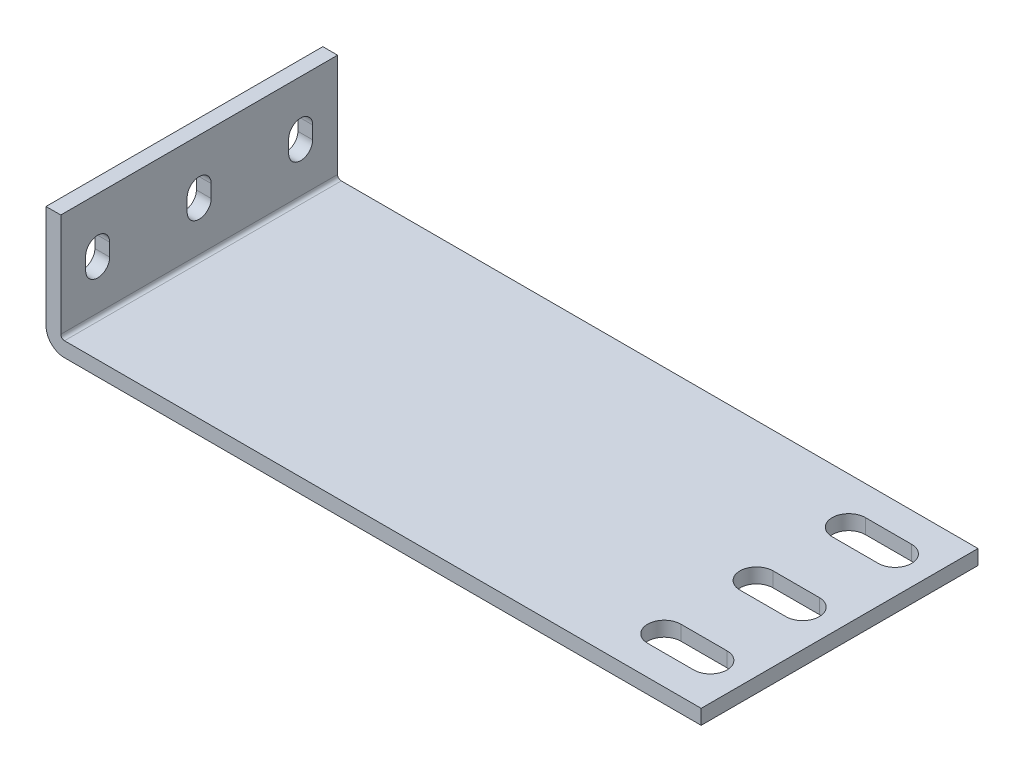
from build123d import *

# Parameters (mm, degrees)
EXTRUDE_1_DEPTH     = 150
CUT_EXTRUDE_1_DEPTH = 150
CUT_EXTRUDE_2_DEPTH = 150


with BuildPart() as part:
    # 草图1 → 凸台-拉伸1 (new body)
    with BuildSketch(Plane.XY):
        with BuildLine():
            Line((0, 0), (0, -56))
            ThreePointArc((0, -56), (2.928932188, -63.071067812), (10, -66))
            Line((10, -66), (355, -66))
            Line((355, -66), (355, -58))
            Line((355, -58), (10, -58))
            ThreePointArc((10, -58), (8.585786438, -57.414213562), (8, -56))
            Line((8, -56), (8, 0))
            Line((8, 0), (0, 0))
        make_face()
    extrude(amount=EXTRUDE_1_DEPTH)

    # 草图2 → 切除-拉伸1 (cut)
    with BuildSketch(Plane.ZY):
        with BuildLine():
            Line((26.5, -26), (26.5, -33))
            ThreePointArc((26.5, -33), (20, -39.5), (13.5, -33))
            Line((13.5, -33), (13.5, -26))
            ThreePointArc((13.5, -26), (20, -19.5), (26.5, -26))
        make_face()
        with BuildLine():
            Line((81.5, -26), (81.5, -33))
            ThreePointArc((81.5, -33), (75, -39.5), (68.5, -33))
            Line((68.5, -33), (68.5, -26))
            ThreePointArc((68.5, -26), (75, -19.5), (81.5, -26))
        make_face()
        with BuildLine():
            Line((136.5, -26), (136.5, -33))
            ThreePointArc((136.5, -33), (130, -39.5), (123.5, -33))
            Line((123.5, -33), (123.5, -26))
            ThreePointArc((123.5, -26), (130, -19.5), (136.5, -26))
        make_face()
    extrude(amount=-CUT_EXTRUDE_1_DEPTH, mode=Mode.SUBTRACT)

    # 草图3 → 切除-拉伸2 (cut)
    with BuildSketch(Plane(origin=(0, -58, 0), x_dir=(1, 0, 0), z_dir=(0, 1, 0))):
        with BuildLine():
            Line((310, -16), (335, -16))
            ThreePointArc((335, -16), (344, -25), (335, -34))
            Line((335, -34), (310, -34))
            ThreePointArc((310, -34), (301, -25), (310, -16))
        make_face()
        with BuildLine():
            Line((310, -66), (335, -66))
            ThreePointArc((335, -66), (344, -75), (335, -84))
            Line((335, -84), (310, -84))
            ThreePointArc((310, -84), (301, -75), (310, -66))
        make_face()
        with BuildLine():
            Line((310, -116), (335, -116))
            ThreePointArc((335, -116), (344, -125), (335, -134))
            Line((335, -134), (310, -134))
            ThreePointArc((310, -134), (301, -125), (310, -116))
        make_face()
    extrude(amount=-CUT_EXTRUDE_2_DEPTH, mode=Mode.SUBTRACT)


solid = part.part
